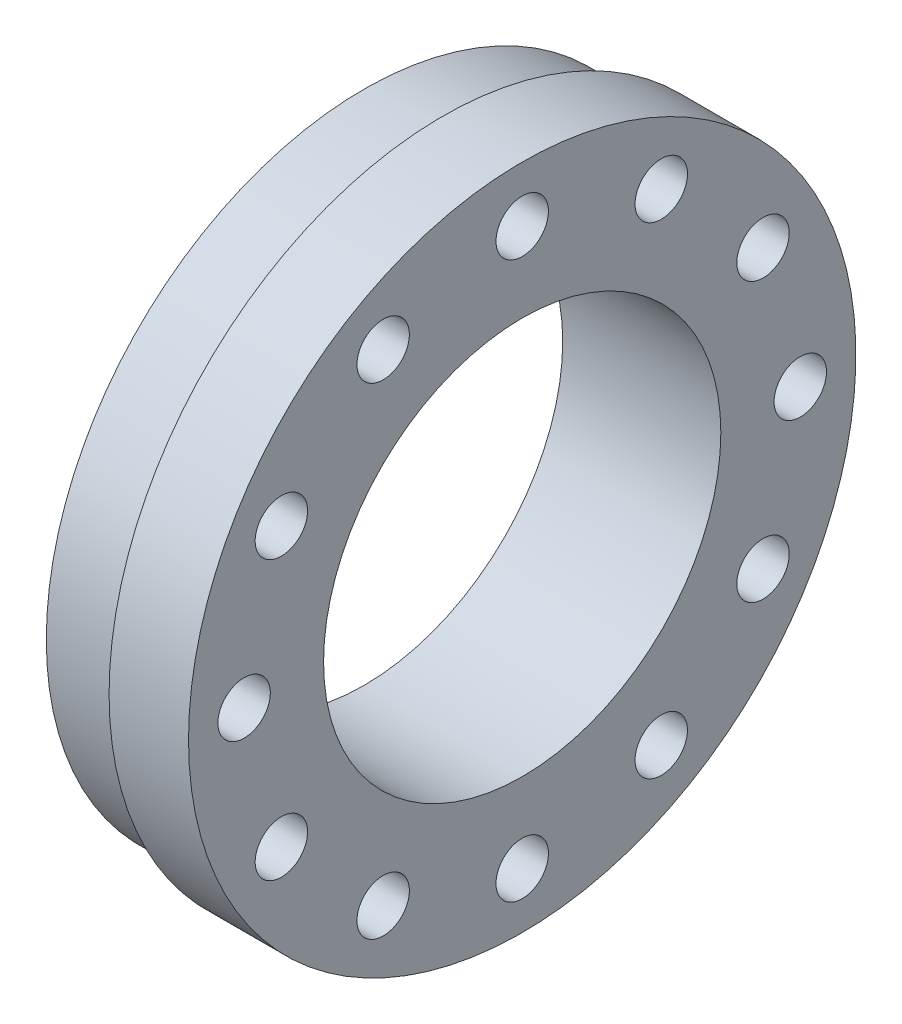
SolidWorks part; units mm, degrees
material "6061 合金"
ref_plane "前视基准面" through (0, 0, 0) normal (0, 0, 1) x (1, 0, 0)
ref_plane "上视基准面" through (0, 0, 0) normal (0, 1, 0) x (1, 0, 0)
ref_plane "右视基准面" through (0, 0, 0) normal (1, 0, 0) x (0, 0, -1)
other "Configuration Table"
sketch "草图1" plane through (0, 0, 0) normal (0, 1, 0) x (1, 0, 0)
  line L0 (-63.9436, 0) -> (3133.2364, 0) construction
  line L1 (0, 12.5) -> (0, 20)
  line L2 (0, 20) -> (4.95, 20)
  line L3 (4.95, 20) -> (4.95, 21)
  line L4 (4.95, 21) -> (9.95, 21)
  line L5 (9.95, 21) -> (9.95, 12.5)
  line L6 (9.95, 12.5) -> (0, 12.5)
  dimension "D1" = 4.95
  dimension "D2" = 5
  dimension "D3" = 25
  dimension "D4" = 40
  dimension "D5" = 42
revolve "旋转1" add sketch "草图1" angle 360 about L0
sketch "草图2" plane through (9.95, 0, 0) normal (1, 0, 0) x (0, 0, -1)
  circle A0 centre (0, 0) radius 17.5 construction
  point P3 (0, 17.5)
  point P4 (-16.6885, 8.6474)
  point P5 (0, 0)
  point P6 (8.75, 15.1554)
  point P7 (15.1554, 8.75)
  point P8 (17.5, 0)
  point P9 (15.1554, -8.75)
  point P10 (8.75, -15.1554)
  point P11 (0, -17.5)
  point P12 (-8.75, -15.1554)
  point P13 (-15.1554, -8.75)
  point P14 (-17.5, 0)
  point P15 (-15.1554, 8.75)
  point P16 (-8.75, 15.1554)
  point P17 (0, 0)
  dimension "D1" = 35
  dimension "D2" = 12
hole_wizard "M4 螺纹孔1" positions "草图2" profile "草图3" tap size "M4" standard "ISO" end condition through all
sketch "草图3" plane through (9.95, 0, 0) normal (0, 1, 0) x (0, 0, -1)
  line L0 (0, 0) -> (0, 9.95)
  line L1 (0, 9.95) -> (1.65, 9.95)
  line L2 (1.65, 9.95) -> (1.65, 0)
  line L5 (1.65, 0) -> (0, 0)
  line L11 (0, -6.35) -> (0, 107.95) construction
  dimension "通孔螺纹孔钻头直径" = 3.3
  dimension "通孔螺纹孔钻头深度" = 9.95
cosmetic thread "孔螺纹线1" parameters "D2"=4
cosmetic thread "孔螺纹线2" parameters "D2"=4
cosmetic thread "孔螺纹线3" parameters "D2"=4
cosmetic thread "孔螺纹线4" parameters "D2"=4
cosmetic thread "孔螺纹线5" parameters "D2"=4
cosmetic thread "孔螺纹线6" parameters "D2"=4
cosmetic thread "孔螺纹线7" parameters "D2"=4
cosmetic thread "孔螺纹线8" parameters "D2"=4
cosmetic thread "孔螺纹线9" parameters "D2"=4
cosmetic thread "孔螺纹线10" parameters "D2"=4
cosmetic thread "孔螺纹线11" parameters "D2"=4
cosmetic thread "孔螺纹线12" parameters "D2"=4
